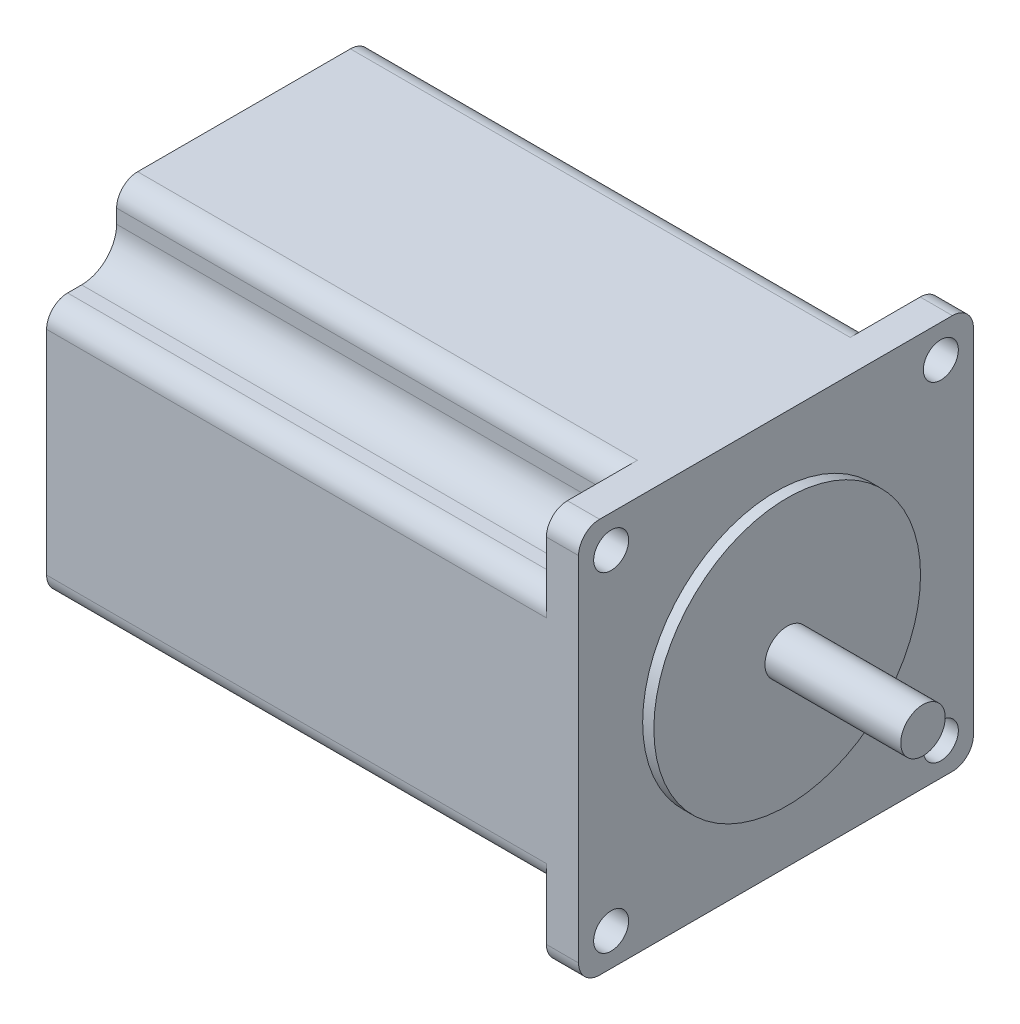
from build123d import *

# Parameters (mm, degrees)
SKETCH_1_W               = 56.4
SKETCH_1_H               = 56.4
EXTRUDE_1_DEPTH          = 76
SKETCH_2_R               = 19.05
EXTRUDE_2_DEPTH          = 1.6
SKETCH_3_R               = 3.175
EXTRUDE_3_DEPTH          = 19.4
FILLET_1_R               = 3
CUT_EXTRUDE_1_DEPTH      = 71.4
SKETCH_5_R               = 2.5
CUT_EXTRUDE_2_DEPTH      = 5
PATTERN_CIRCULAR_3_COUNT = 4
FILLET_2_R               = 3


with BuildPart() as part:
    # 草图1 → 凸台-拉伸1 (new body)
    with BuildSketch(Plane(origin=(0, 0, 0), x_dir=(0, 0, -1), z_dir=(1, 0, 0))):
        Rectangle(SKETCH_1_W, SKETCH_1_H)
    extrude(amount=EXTRUDE_1_DEPTH)

    # 草图2 → 凸台-拉伸2 (add)
    with BuildSketch(Plane(origin=(76, 0, 0), x_dir=(0, 0, -1), z_dir=(1, 0, 0))):
        with Locations(Location((0, 0, 0), (0, 0, 180))):
            Circle(SKETCH_2_R)
    extrude(amount=EXTRUDE_2_DEPTH)

    # 草图3 → 凸台-拉伸3 (add)
    with BuildSketch(Plane(origin=(77.6, 0, 0), x_dir=(0, 0, -1), z_dir=(1, 0, 0))):
        Circle(SKETCH_3_R)
    extrude(amount=EXTRUDE_3_DEPTH)

    # 圆角1
    fillet_1_edges = [part.edges().sort_by_distance(p)[0] for p in [
        (38, -28.2, -28.2),
        (38, -28.2, 28.2),
        (38, 28.2, 28.2),
        (38, 28.2, -28.2),
    ]]
    fillet(fillet_1_edges, radius=FILLET_1_R)

    # 草图4 → 切除-拉伸1 (cut)
    with BuildSketch(Plane.ZY):
        with BuildLine():
            Line((-28.2, 28.2), (-18.2, 28.2))
            Line((-18.2, 28.2), (-18.2, 23.2))
            ThreePointArc((-18.2, 23.2), (-19.664466094, 19.664466094), (-23.2, 18.2))
            Line((-23.2, 18.2), (-28.2, 18.2))
            Line((-28.2, 18.2), (-28.2, 28.2))
        make_face()
    cut_extrude_1 = extrude(amount=-CUT_EXTRUDE_1_DEPTH, mode=Mode.SUBTRACT)

    # 草图5 → 切除-拉伸2 (cut)
    with BuildSketch(Plane.ZY.offset(-71.4)):
        with Locations((-23.55, 23.55)):
            Circle(SKETCH_5_R)
    cut_extrude_2 = extrude(amount=-CUT_EXTRUDE_2_DEPTH, mode=Mode.SUBTRACT)

    # 阵列(圆周)3: 切除-拉伸1, 切除-拉伸2 ×4 about axis
    pattern_circular_3_axis = Axis((0, 0, 0), (1, 0, 0))
    add([cut_extrude_1.rotate(pattern_circular_3_axis, i * 360 / PATTERN_CIRCULAR_3_COUNT) for i in range(1, PATTERN_CIRCULAR_3_COUNT)], mode=Mode.SUBTRACT)
    add([cut_extrude_2.rotate(pattern_circular_3_axis, i * 360 / PATTERN_CIRCULAR_3_COUNT) for i in range(1, PATTERN_CIRCULAR_3_COUNT)], mode=Mode.SUBTRACT)

    # 圆角2
    fillet_2_edges = [part.edges().sort_by_distance(p)[0] for p in [
        (35.7, 28.2, 18.2),
        (35.7, 18.2, 28.2),
        (35.7, 18.2, -28.2),
        (35.7, 28.2, -18.2),
        (35.7, -28.2, -18.2),
        (35.7, -18.2, -28.2),
        (35.7, -18.2, 28.2),
        (35.7, -28.2, 18.2),
    ]]
    fillet(fillet_2_edges, radius=FILLET_2_R)


solid = part.part
